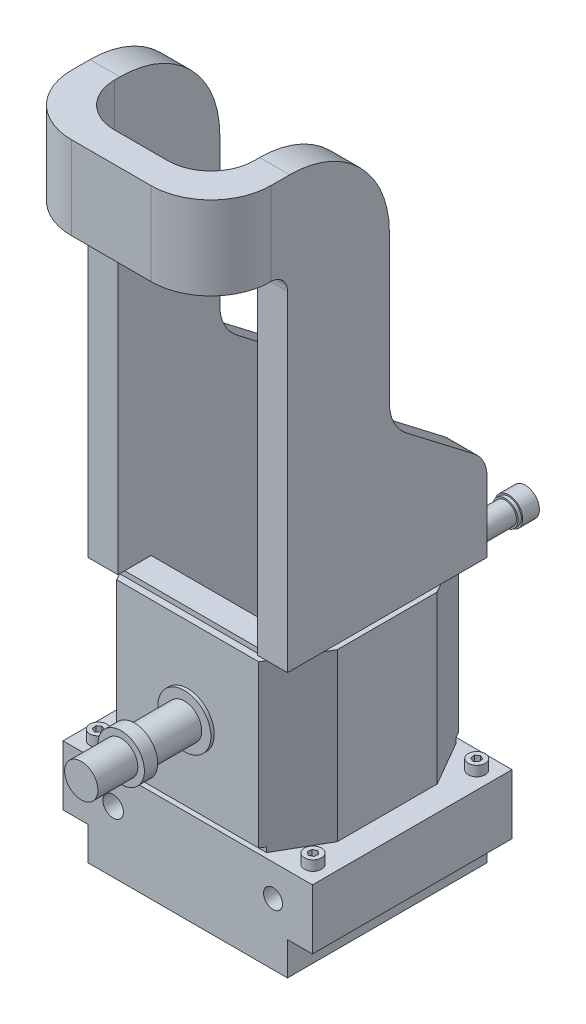
SolidWorks part; units mm, degrees
ref_plane "Front Plane" through (0, 0, 0) normal (0, 0, 1) x (1, 0, 0)
ref_plane "Top Plane" through (0, 0, 0) normal (0, 1, 0) x (1, 0, 0)
ref_plane "Right Plane" through (0, 0, 0) normal (1, 0, 0) x (0, 0, -1)
other "Configuration Table"
sketch "Sketch1" plane through (0, 0, 0) normal (0, 1, 0) x (1, 0, 0)
  line L1 (-20, 20) -> (20, 20)
  line L2 (-20, 20) -> (-20, -20)
  line L3 (-20, -20) -> (20, -20)
  line L4 (20, 20) -> (20, -20)
  line L5 (-20, 20) -> (20, -20) construction
  line L6 (-20, -20) -> (20, 20) construction
  line L7 (30, -30) -> (-30, -30)
  line L8 (30, -30) -> (30, 30)
  line L9 (30, 30) -> (-30, 30)
  line L10 (-30, -30) -> (-30, 30)
  line L11 (30, -30) -> (-30, 30) construction
  line L12 (30, 30) -> (-30, -30) construction
  point P0 (0, 0)
  point P6 (0, 0)
  dimension "D1" = 40
  dimension "D2" = 40
  dimension "D3" = 60
  dimension "D4" = 60
extrude "Boss-Extrude1" add sketch "Sketch1" along normal blind 10
sketch "Sketch2" plane through (0, 10, 0) normal (0, 1, 0) x (1, 0, 0)
  line L1 (37.5, -30) -> (-37.5, -30)
  line L2 (37.5, -30) -> (37.5, 30)
  line L3 (37.5, 30) -> (-37.5, 30)
  line L4 (-37.5, -30) -> (-37.5, 30)
  line L5 (37.5, -30) -> (-37.5, 30) construction
  line L6 (37.5, 30) -> (-37.5, -30) construction
  point P0 (0, 0)
  dimension "D1" = 75
  dimension "D2" = 60
extrude "Boss-Extrude2" add sketch "Sketch2" along normal blind 18
sketch "Sketch4" plane through (0, 28, 0) normal (0, 1, 0) x (1, 0, 0)
  line L0 (37.5, 30) -> (-37.5, 30) construction
  line L1 (-30, 30) -> (30, 30)
  line L2 (-30, 30) -> (-30, -30)
  line L3 (-30, -30) -> (30, -30)
  line L4 (30, 30) -> (30, -30)
  line L5 (-37.5, -30) -> (37.5, -30) construction
  line L6 (-37.5, 30) -> (-37.5, -30) construction
  line L7 (37.5, -30) -> (37.5, 30) construction
  dimension "D1" = 7.5
  dimension "D2" = 7.5
extrude "Boss-Extrude3" add sketch "Sketch4" along normal blind 50
chamfer "Chamfer1" distance 15 angle 30 2 edges at (-30, 53, 30) (30, 53, -30)
chamfer "Chamfer2" distance 15 angle 30 2 edges at (30, 53, 30) (-30, 53, -30)
sketch "Sketch5" plane through (0, 0, -30) normal (0, 0, -1) x (-1, 0, 0)
  line L0 (0, 5.5) -> (0, -5.5) construction
  line L1 (-15.225, 70.9554) -> (15.225, 70.9554)
  line L2 (-15.225, 70.9554) -> (-15.225, 48.5838)
  line L3 (-15.225, 48.5838) -> (15.225, 48.5838)
  line L4 (15.225, 70.9554) -> (15.225, 48.5838)
  line L5 (-15.225, 70.9554) -> (15.225, 48.5838) construction
  line L6 (-15.225, 48.5838) -> (15.225, 70.9554) construction
  point P0 (0, 59.7696)
extrude "Cut-Extrude1" cut sketch "Sketch5" against normal blind 20
sketch "Sketch6" plane through (0, 28, 0) normal (0, 1, 0) x (1, 0, 0)
  line L0 (-24.8129, 28.5) -> (23.7963, 28.5)
  line L1 (23.7963, 28.5) -> (23.7963, 32.3813)
  line L2 (23.7963, 32.3813) -> (-26.9384, 32.3813)
  line L3 (-26.9384, 32.3813) -> (-24.8129, 28.5)
  line L4 (-25.8756, -28.5) -> (26.5687, -28.5)
  line L5 (26.5687, -28.5) -> (25.3673, -32.1965)
  line L6 (25.3673, -32.1965) -> (-25.8756, -32.1965)
  line L7 (-25.8756, -32.1965) -> (-25.8756, -28.5)
  line L8 (-37.5, -30) -> (-21.3397, -30) construction
  line L9 (-21.3397, 30) -> (-37.5, 30) construction
  dimension "D1" = 1.5
  dimension "D2" = 1.5
extrude "Cut-Extrude2" cut sketch "Sketch6" along normal blind 1.5
sketch "Sketch7" plane through (0, 28, 0) normal (0, 1, 0) x (1, 0, 0)
  line L1 (33.4846, 24.0938) -> (33.3275, 25.3987)
  line L2 (33.3275, 25.3987) -> (32.1189, 25.9151)
  line L3 (32.1189, 25.9151) -> (31.0674, 25.1266)
  line L4 (31.0674, 25.1266) -> (31.2245, 23.8217)
  line L5 (31.2245, 23.8217) -> (32.4331, 23.3053)
  line L6 (32.4331, 23.3053) -> (33.4846, 24.0938)
  circle A0 centre (32.276, 24.6102) radius 2.5475
  circle A1 centre (32.276, 24.6102) radius 1.1382 construction
extrude "Boss-Extrude4" add sketch "Sketch7" along normal blind 3
mirror "Mirror3" about plane through (0, 0, 0) normal (1, 0, 0) of "Boss-Extrude4"
mirror "Mirror4" about plane through (0, 0, 0) normal (0, 0, 1) of "Mirror3", "Boss-Extrude4"
sketch "Sketch8" plane through (0, 0, -30) normal (0, 0, -1) x (-1, 0, 0)
  circle A0 centre (-25.6492, 18.5167) radius 2.8556
  circle A1 centre (22.4055, 18.5167) radius 3.077
extrude "Cut-Extrude3" cut sketch "Sketch8" against normal up to next
sketch "Sketch10" plane through (0, 78, 0) normal (0, 1, 0) x (1, 0, 0)
  line L0 (-30, 15) -> (-30, -15) construction
  line L1 (-21, 20) -> (21, 20)
  line L2 (-21, 20) -> (-21, -20)
  line L3 (-21, -20) -> (21, -20)
  line L4 (21, 20) -> (21, -20)
  line L5 (-21, 20) -> (21, -20) construction
  line L6 (-21, -20) -> (21, 20) construction
  line L7 (21.3397, 30) -> (-21.3397, 30) construction
  point P0 (0, 0)
  dimension "D1" = 9
  dimension "D2" = 10
extrude "Cut-Extrude4" cut sketch "Sketch10" against normal blind 40
sketch "Sketch11" plane through (30, 0, 0) normal (1, 0, 0) x (0, 0, -1)
  line L0 (-30, 79.5) -> (-30, 183.7925)
  line L1 (-30, 183.7925) -> (0.6405, 183.7925)
  line L2 (0.6405, 183.7925) -> (0.6405, 127.9402)
  line L3 (0.6405, 127.9402) -> (30, 105.4081)
  line L4 (30, 105.4081) -> (30, 79.5)
  line L5 (30, 79.5) -> (-30, 79.5)
  line L6 (-15, 78) -> (15, 78) construction
  line L7 (-30, 29.5) -> (-30, 78) construction
  line L8 (30, 78) -> (30, 29.5) construction
  dimension "D1" = 1.5
extrude "Boss-Extrude5" add sketch "Sketch11" against normal blind 9
sketch "Sketch12" plane through (0, 78, 0) normal (0, 1, 0) x (1, 0, 0)
  line L1 (28.0473, -27.9549) -> (-28.0473, -27.9549)
  line L2 (28.0473, -27.9549) -> (28.0473, 27.9549)
  line L3 (28.0473, 27.9549) -> (-28.0473, 27.9549)
  line L4 (-28.0473, -27.9549) -> (-28.0473, 27.9549)
  line L5 (28.0473, -27.9549) -> (-28.0473, 27.9549) construction
  line L6 (28.0473, 27.9549) -> (-28.0473, -27.9549) construction
  line L7 (21, -20) -> (-21, -20)
  line L8 (21, -20) -> (21, 20)
  line L9 (21, 20) -> (-21, 20)
  line L10 (-21, -20) -> (-21, 20)
  line L11 (21, -20) -> (-21, 20) construction
  line L12 (21, 20) -> (-21, -20) construction
  point P0 (0, 0)
  point P6 (0, 0)
extrude "Boss-Extrude6" add sketch "Sketch12" along normal blind 1.5
mirror "Mirror5" about plane through (0, 0, 0) normal (1, 0, 0) of "Boss-Extrude5"
sketch "Sketch13" plane through (0, 183.7925, 0) normal (0, 1, 0) x (1, 0, 0)
  line L0 (-30, 0.6405) -> (-21, 0.6405)
  line L1 (-21, 0.6405) -> (-21, -30)
  line L2 (-21, -30) -> (-21, -44)
  line L3 (30, 0.6405) -> (21, 0.6405)
  line L4 (21, 0.6405) -> (21, -30)
  line L5 (21, -30) -> (30, -30) construction
  line L6 (21, 0.6405) -> (21, -30) construction
  line L7 (21, -30) -> (21, -44)
  line L8 (21, -44) -> (-21, -44)
  line L9 (-30, 0.6405) -> (-30, -53)
  line L10 (-30, -53) -> (30, -53)
  line L11 (30, -53) -> (30, 0.6405)
  dimension "D1" = 14
  dimension "D2" = 9
extrude "Boss-Extrude7" add sketch "Sketch13" along normal blind 25
fillet "Fillet1" radius 18 2 edges at (-30, 196.2925, 53) (30, 196.2925, 53)
fillet "Fillet2" radius 13 2 edges at (21, 196.2925, 44) (-21, 196.2925, 44)
fillet "Fillet3" radius 13 2 edges at (25.5, 127.9402, -0.6405) (-25.5, 127.9402, -0.6405)
fillet "Fillet4" radius 10 2 edges at (25.5, 105.4081, -30) (-25.5, 105.4081, -30)
fillet "Fillet6" radius 5 2 edges at (-25.5, 183.7925, 30) (25.5, 183.7925, 30)
fillet "Fillet7" radius 30 2 edges at (25.5, 208.7925, -0.6405) (-25.5, 208.7925, -0.6405)
sketch "Sketch14" plane through (0, 0, -30) normal (0, 0, -1) x (-1, 0, 0)
  circle A0 centre (-25.5, 83.8128) radius 3.333
  circle A1 centre (25.6692, 83.8128) radius 3.4335
extrude "Boss-Extrude8" add sketch "Sketch14" along normal blind 10
sketch "Sketch15" plane through (0, 0, -40) normal (0, 0, -1) x (-1, 0, 0)
  circle A0 centre (-25.5, 83.8128) radius 3.8054
  circle A1 centre (25.6692, 83.8128) radius 3.9569
extrude "Boss-Extrude9" add sketch "Sketch15" along normal blind 1
sketch "Sketch16" plane through (0, 0, -41) normal (0, 0, -1) x (-1, 0, 0)
  circle A0 centre (-25.5, 83.8128) radius 4.2306
  circle A1 centre (25.6692, 83.8128) radius 4.414
extrude "Boss-Extrude10" add sketch "Sketch16" along normal blind 5
sketch "Sketch17" plane through (0, 0, -46) normal (0, 0, -1) x (-1, 0, 0)
  line L1 (-23.577, 82.5576) -> (-23.4514, 84.8506)
  line L2 (-23.4514, 84.8506) -> (-25.3744, 86.1058)
  line L3 (-25.3744, 86.1058) -> (-27.423, 85.0681)
  line L4 (-27.423, 85.0681) -> (-27.5486, 82.7751)
  line L5 (-27.5486, 82.7751) -> (-25.6256, 81.5198)
  line L6 (-25.6256, 81.5198) -> (-23.577, 82.5576)
  line L7 (27.6479, 82.5576) -> (27.7457, 84.8987)
  line L8 (27.7457, 84.8987) -> (25.767, 86.154)
  line L9 (25.767, 86.154) -> (23.6906, 85.0681)
  line L10 (23.6906, 85.0681) -> (23.5928, 82.7269)
  line L11 (23.5928, 82.7269) -> (25.5715, 81.4716)
  line L12 (25.5715, 81.4716) -> (27.6479, 82.5576)
  circle A0 centre (-25.5, 83.8128) radius 1.9888 construction
  circle A1 centre (25.6692, 83.8128) radius 2.0293 construction
extrude "Cut-Extrude5" cut sketch "Sketch17" against normal blind 3
sketch "Sketch18" plane through (0, 0, 30) normal (0, 0, 1) x (1, 0, 0)
  line L0 (0, -33) -> (0, 33) construction
  circle A0 centre (0, 52.3962) radius 7.9786
extrude "Boss-Extrude11" add sketch "Sketch18" along normal blind 1
sketch "Sketch19" plane through (0, 0, 31) normal (0, 0, 1) x (1, 0, 0)
  circle A0 centre (0, 52.3962) radius 5.2211
extrude "Boss-Extrude12" add sketch "Sketch19" along normal blind 15
sketch "Sketch20" plane through (0, 0, 46) normal (0, 0, 1) x (1, 0, 0)
  circle A0 centre (0, 52.3962) radius 6.9871
extrude "Boss-Extrude13" add sketch "Sketch20" along normal blind 4
sketch "Sketch21" plane through (0, 0, 50) normal (0, 0, 1) x (1, 0, 0)
  circle A0 centre (0, 52.3962) radius 5.0098
extrude "Boss-Extrude14" add sketch "Sketch21" along normal blind 12
sketch "Sketch22" plane through (0, 0, 20) normal (0, 0, -1) x (-1, 0, 0)
  line L0 (0, 33) -> (0, -33) construction
  circle A0 centre (0, 59.5198) radius 4.8663
extrude "Boss-Extrude15" add sketch "Sketch22" along normal blind 12
sketch "Sketch23" plane through (0, 0, 8) normal (0, 0, -1) x (-1, 0, 0)
  line L1 (2.679, 57.5972) -> (3.0045, 60.8786)
  line L2 (3.0045, 60.8786) -> (0.3255, 62.8012)
  line L3 (0.3255, 62.8012) -> (-2.679, 61.4424)
  line L4 (-2.679, 61.4424) -> (-3.0045, 58.161)
  line L5 (-3.0045, 58.161) -> (-0.3255, 56.2384)
  line L6 (-0.3255, 56.2384) -> (2.679, 57.5972)
  circle A0 centre (0, 59.5198) radius 6.4414
  circle A1 centre (0, 59.5198) radius 2.8557 construction
extrude "Boss-Extrude16" add sketch "Sketch23" along normal blind 6
sketch "Sketch24" plane through (0, 0, -30) normal (0, 0, -1) x (-1, 0, 0)
  line L0 (0, 33) -> (0, -33) construction
  circle A0 centre (0, 38.1294) radius 3.6264
extrude "Boss-Extrude17" add sketch "Sketch24" along normal blind 6
sketch "Sketch25" plane through (0, 0, -36) normal (0, 0, -1) x (-1, 0, 0)
